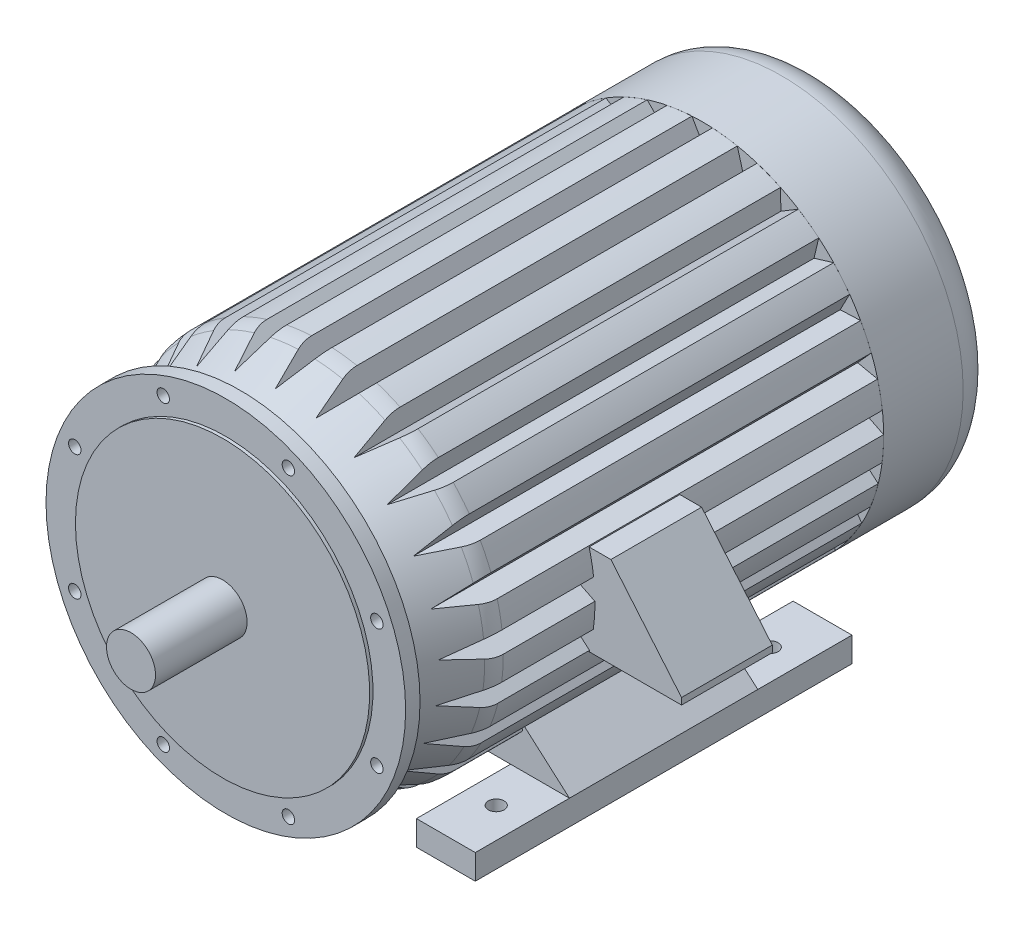
SolidWorks part; units mm, degrees
ref_plane "Front Plane" through (0, 0, 0) normal (0, 0, 1) x (1, 0, 0)
ref_plane "Top Plane" through (0, 0, 0) normal (0, 1, 0) x (1, 0, 0)
ref_plane "Right Plane" through (0, 0, 0) normal (1, 0, 0) x (0, 0, -1)
sketch "Sketch1" plane through (0, 0, 0) normal (0, 0, 1) x (1, 0, 0)
  circle A0 centre (0, 0) radius 37.5
  dimension "D" = 75
extrude "Extrude1" add sketch "Sketch1" against normal blind 140
ref_plane "Plane1" through (0, 0, -1050) normal (0, 0, 1) x (1, 0, 0)
sketch "Sketch3" plane through (0, 0, -140) normal (0, 0, -1) x (-1, 0, 0)
  circle A0 centre (0, 0) radius 225
  dimension "N" = 450
extrude "Extrude2" add sketch "Sketch3" along normal blind 5
sketch "Sketch4" plane through (0, 0, -145) normal (0, 0, -1) x (-1, 0, 0)
  circle A0 centre (0, 0) radius 275
extrude "Extrude3" add sketch "Sketch4" along normal blind 22
ref_plane "Plane6" through (0, 0, -167) normal (0, 0, 1) x (1, 0, 0)
sketch "Sketch5" plane through (0, 0, -167) normal (0, 0, 1) x (1, 0, 0)
  circle A0 centre (0, 0) radius 277.5
extrude "Extrude4" add sketch "Sketch5" along normal up to surface (883 mm away)
sketch "Sketch7" plane through (0, 0, -167) normal (0, 0, -1) x (-1, 0, 0)
  circle A0 centre (0, 0) radius 225
extrude "Cut-Extrude2" cut sketch "Sketch7" along normal through all draft 25 flip side to cut
sketch "Sketch6" plane through (0, 0, -145) normal (0, 0, 1) x (1, 0, 0)
  line L0 (0, 0) -> (0, 250) construction
  line L1 (0, 250) -> (0, 0) construction
  line L2 (0, 0) -> (-95.6709, 230.9699) construction
  circle A0 centre (0, 0) radius 250 construction
  circle A1 centre (-95.6709, 230.9699) radius 9.5
extrude "Cut-Extrude1" cut sketch "Sketch6" against normal blind 22
pattern_circular "CirPattern1" count 8 over 360 about axis through (0, 0, 0) along (0, 0, 1) of "Cut-Extrude1"
fillet "Fillet1" radius 55 2 edges at (277.5, 0, -1050) (-277.5, 0, -279.5866)
ref_plane "Plane2" through (0, 0, -873.4) normal (0, 0, -1) x (-1, 0, 0)
sketch "Sketch8" plane through (0, 0, -873.4) normal (0, 0, -1) x (-1, 0, 0)
  circle A0 centre (0, 0) radius 277.6
extrude "Extrude5" add sketch "Sketch8" along normal blind 121.6
sketch "Sketch9" plane through (0, 0, -873.4) normal (0, 0, -1) x (-1, 0, 0)
  line L1 (0, 250) -> (23.8157, 291.25)
  line L2 (23.8157, 291.25) -> (-23.8157, 291.25)
  line L3 (-23.8157, 291.25) -> (0, 250)
  circle A0 centre (0, 0) radius 277.5 construction
  circle A1 centre (0, 277.5) radius 27.5 construction
extrude "Cut-Extrude3" cut sketch "Sketch9" against normal blind 696.4
pattern_circular "CirPattern2" count 25 over 360 about axis through (0, 0, 0) along (0, 0, 1) of "Cut-Extrude3"
sketch "Sketch10" plane through (0, 0, 0) normal (1, 0, 0) x (0, 0, -1)
  line L1 (431.9, 69.375) -> (570.65, 69.375)
  line L2 (431.9, 69.375) -> (431.9, -69.375)
  line L3 (431.9, -69.375) -> (570.65, -69.375)
  line L4 (570.65, 69.375) -> (570.65, -69.375)
  line L5 (873.4, 0) -> (291.7798, 0) construction
  line L6 (167, -275) -> (167, 275) construction
extrude "Extrude6" add sketch "Sketch10" along normal blind 410
chamfer "Chamfer1" distance 128.75 angle 40 1 edges at (410, 69.375, -501.275)
ref_plane "Plane3" through (0, 0, -608.5) normal (0, 0, 1) x (1, 0, 0)
ref_plane "Plane4" through (0, -280, 0) normal (0, 1, 0) x (-1, 0, 0)
sketch "Sketch11" plane through (0, -280, 0) normal (0, 1, 0) x (-1, 0, 0)
  line L0 (184.1897, -539.5) -> (-183.3621, -539.5) construction
  line L1 (225, -140) -> (-225, -140) construction
  line L3 (0, 0) -> (0, -307.658) construction
  line L4 (275, -827.5) -> (185, -827.5)
  line L5 (-275, -251.5) -> (-185, -251.5)
  line L6 (-275, -251.5) -> (-275, -827.5)
  line L7 (-275, -827.5) -> (-185, -827.5)
  line L8 (-185, -251.5) -> (-185, -827.5)
  line L9 (185, -251.5) -> (185, -827.5)
  line L10 (275, -251.5) -> (185, -251.5)
  line L11 (275, -251.5) -> (275, -827.5)
  circle A0 centre (-228.5, -330) radius 12
  circle A1 centre (-228.5, -749) radius 12
  circle A2 centre (228.5, -749) radius 12
  circle A3 centre (228.5, -330) radius 12
extrude "Extrude7" add sketch "Sketch11" along normal blind 38
ref_plane "Plane5" through (0, 0, -539.5) normal (0, 0, 1) x (1, 0, 0)
sketch "Sketch12" plane through (0, 0, -539.5) normal (0, 0, 1) x (1, 0, 0)
  line L0 (275, -242) -> (0, 0)
  line L1 (0, 0) -> (-275, -242)
  line L2 (-275, -242) -> (275, -242)
extrude "Extrude8" add sketch "Sketch12" along normal mid plane 288
equation "\"D1@Cut-Extrude1\" = \"LA@Extrude3\""
equation "\"D1@Fillet1\" = \"P@Sketch4\" / 10"
equation "\"D1@Sketch7\" = \"M@Sketch6\" -  ( \"P@Sketch4\" - \"M@Sketch6\" )"
equation "\"D1@Plane2\" = ( \"L@Plane1\" - \"E@Extrude1\" - \"T@Extrude2\" - \"LA@Extrude3\" )  / 5"
equation "\"D1@Sketch8\" = \"AC@Sketch5\" + 0.2"
equation "\"D1@Extrude5\" = \"D1@Plane2\" - \"D1@Fillet1\""
equation "\"D1@Sketch9\" = \"AC@Sketch5\" "
equation "\"D2@Sketch9\" = \"D1@Fillet1\""
equation "\"D1@Cut-Extrude3\" = \"L@Plane1\" - \"E@Extrude1\" - \"T@Extrude2\" - \"LA@Extrude3\" - \"D1@Plane2\" - 10"
equation "\"D2@Sketch10\" = \"D1@Sketch10\" / 2"
equation "\"D3@Sketch10\" = \"D1@Sketch10\""
equation "\"D1@Plane3\" = \"L@Plane1\" / 2 +  \"E@Extrude1\" / 2 + \"T@Extrude2\" / 2 + \"LA@Extrude3\"   / 2 "
equation "\"D6@Sketch11\" = \"BB@Sketch11\" / 2"
equation "\"D1@Plane5\" = \"BB@Sketch11\" / 2"
equation "\"D1@Extrude8\" = \"BB@Sketch11\" / 2"
equation "\"D1@Chamfer1\" = \"D1@Sketch10\" - 10"
equation "\"D1@Plane6\" = \"E@Extrude1\" + \"T@Extrude2\" + \"LA@Extrude3\""
equation "\"D1@Sketch10\" = \"AC@Sketch5\" / 4"
equation "\"D4@Sketch10\" = (  \"L@Plane1\" - \"E@Extrude1\" - \"LA@Extrude3\" - \"T@Extrude2\" )   * 0.3"
